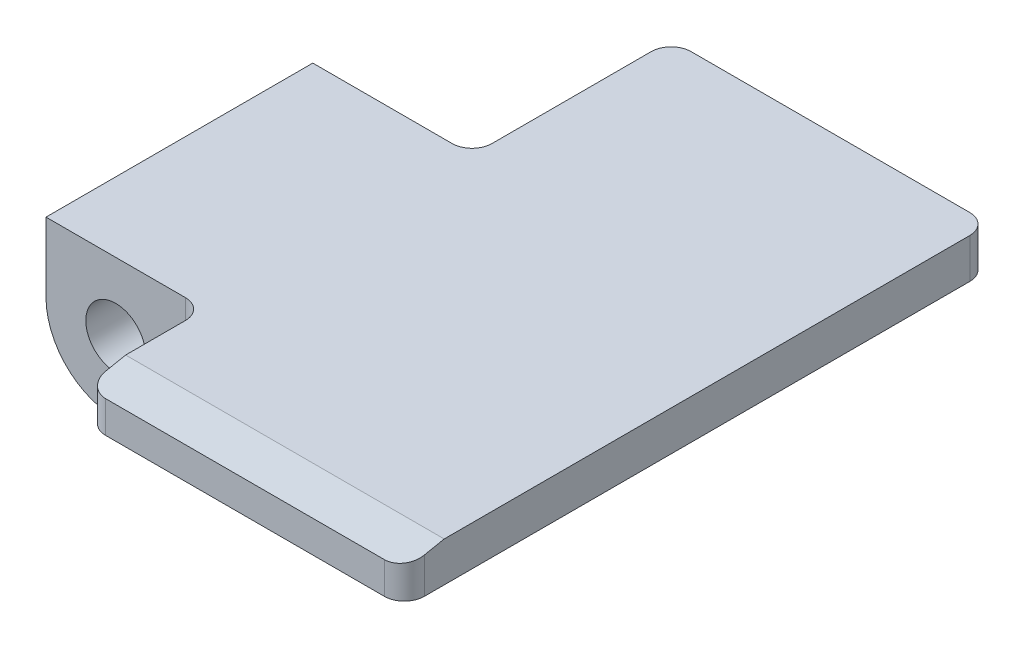
from build123d import *

# Parameters (mm, degrees)
SKETCH1_R           = 1.75
BOSS_EXTRUDE1_DEPTH = 6.7
SKETCH2_R           = 0.75
CUT_EXTRUDE1_DEPTH  = 8.142478561
SKETCH3_W           = 12
SKETCH3_H           = 6.7
BOSS_EXTRUDE2_DEPTH = 1
BOSS_EXTRUDE3_START = -6.7
BOSS_EXTRUDE3_DEPTH = 6.7
SKETCH5_W           = 8
SKETCH5_H           = 1
BOSS_EXTRUDE4_DEPTH = 3
SKETCH6_W           = 8
SKETCH6_H           = 1
BOSS_EXTRUDE5_DEPTH = 5
CHAMFER1_SIZE       = 1
CHAMFER1_SIZE2      = 0.2
FILLET1_R           = 0.5


with BuildPart() as part:
    # Sketch1 → Boss-Extrude1 (new body)
    with BuildSketch(Plane.XY):
        Circle(SKETCH1_R)
    extrude(amount=BOSS_EXTRUDE1_DEPTH)

    # Sketch2 → Cut-Extrude1 (cut, through all)
    with BuildSketch(Plane.XY.offset(6.7)):
        Circle(SKETCH2_R)
    extrude(amount=-CUT_EXTRUDE1_DEPTH, mode=Mode.SUBTRACT)

    # Sketch3 → Boss-Extrude2 (add)
    with BuildSketch(Plane(origin=(0, 1.75, 0), x_dir=(1, 0, 0), z_dir=(0, 1, 0))):
        with Locations((4.25, -3.35)):
            Rectangle(SKETCH3_W, SKETCH3_H)
    extrude(amount=-BOSS_EXTRUDE2_DEPTH)

    # Sketch4 → Boss-Extrude3 (add)
    with BuildSketch(Plane.XY.offset(6.7).offset(BOSS_EXTRUDE3_START)):
        with BuildLine():
            Line((-1.75, 0.75), (-1.75, 0))
            ThreePointArc((-1.75, 0), (-1.707262861, 0.384387205), (-1.58113883, 0.75))
            Line((-1.58113883, 0.75), (-1.75, 0.75))
        make_face()
    extrude(amount=BOSS_EXTRUDE3_DEPTH)

    # Sketch5 → Boss-Extrude4 (add)
    with BuildSketch(Plane.XY.offset(6.7)):
        with Locations((6.25, 1.25)):
            Rectangle(SKETCH5_W, SKETCH5_H)
    extrude(amount=BOSS_EXTRUDE4_DEPTH)

    # Sketch6 → Boss-Extrude5 (add)
    with BuildSketch(Plane(origin=(0, 0, 0), x_dir=(-1, 0, 0), z_dir=(0, 0, -1))):
        with Locations((-6.25, 1.25)):
            Rectangle(SKETCH6_W, SKETCH6_H)
    extrude(amount=BOSS_EXTRUDE5_DEPTH)

    # Chamfer1
    chamfer1_edges = [part.edges().sort_by_distance(p)[0] for p in [
        (6.25, 1.75, 9.7),
    ]]
    chamfer1_side = [part.faces().sort_by_distance(p)[0] for p in [
        (5.136426593, 1.75, 2.535595568),
    ]]
    chamfer(chamfer1_edges, length=CHAMFER1_SIZE, length2=CHAMFER1_SIZE2, reference=chamfer1_side[0])

    # Fillet1
    fillet1_edges = [part.edges().sort_by_distance(p)[0] for p in [
        (2.25, 1.25, 6.7),
        (10.25, 1.15, 9.7),
        (2.25, 1.25, 0),
        (10.25, 1.25, -5),
        (2.25, 1.25, -5),
        (2.25, 1.15, 9.7),
    ]]
    fillet(fillet1_edges, radius=FILLET1_R)


solid = part.part
